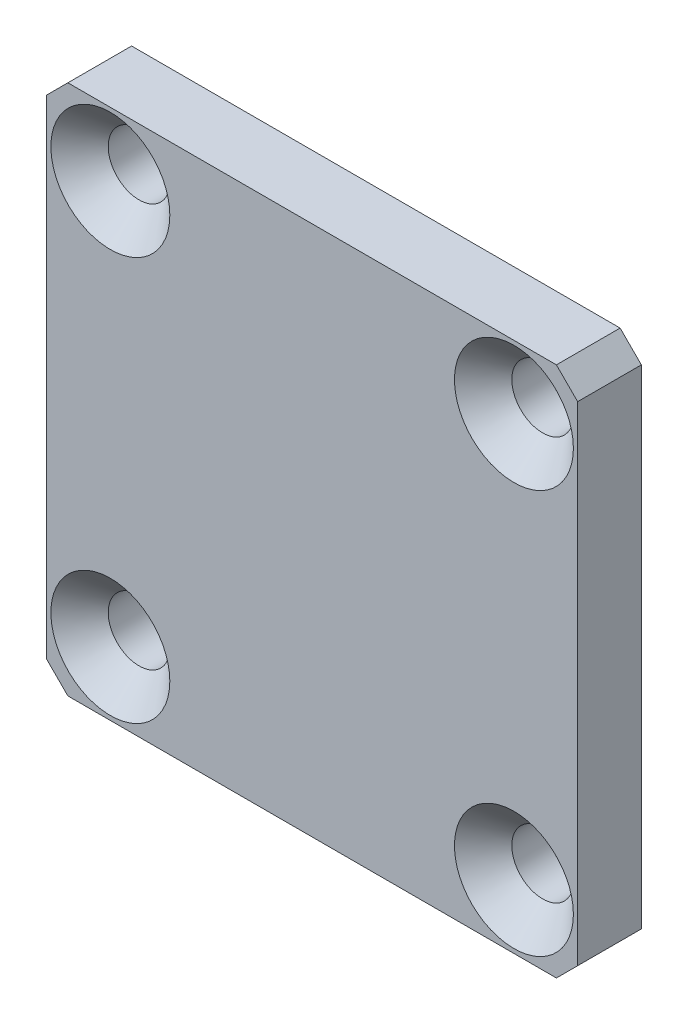
SolidWorks part; units mm, degrees
material "6061Al"
ref_plane "前视基准面" through (0, 0, 0) normal (0, 0, 1) x (1, 0, 0)
ref_plane "上视基准面" through (0, 0, 0) normal (0, 1, 0) x (1, 0, 0)
ref_plane "右视基准面" through (0, 0, 0) normal (1, 0, 0) x (0, 0, -1)
sketch "草图1" plane through (0, 0, 0) normal (0, 0, 1) x (1, 0, 0)
  line L1 (-25, -25) -> (25, -25)
  line L2 (-25, -25) -> (-25, 25)
  line L3 (-25, 25) -> (25, 25)
  line L4 (25, -25) -> (25, 25)
  line L5 (-25, -25) -> (25, 25) construction
  line L6 (-25, 25) -> (25, -25) construction
  point P0 (0, 0)
  dimension "D1" = 50
  dimension "D2" = 50
extrude "凸台-拉伸1" add sketch "草图1" along normal mid plane 6
sketch "草图2" plane through (0, 0, 3) normal (0, 0, 1) x (1, 0, 0)
  circle A0 centre (0, 0) radius 20
  dimension "D1" = 40
extrude "切除-拉伸1" [suppressed] cut sketch "草图2" against normal through all
hole_wizard "M5 六角凹锥坑螺钉的锥形沉头孔1" positions "草图6" profile "草图5" countersink size "M5" standard "ISO" end condition through all
sketch "草图6" plane through (0, 0, 3) normal (0, 0, 1) x (1, 0, 0)
  line L1 (-19, -19) -> (19, -19)
  line L2 (-19, -19) -> (-19, 19)
  line L3 (-19, 19) -> (19, 19)
  line L4 (19, -19) -> (19, 19)
  line L5 (-19, -19) -> (19, 19) construction
  line L6 (-19, 19) -> (19, -19) construction
  line L7 (-25, 25) -> (-25, -25) construction
  point P0 (-19, 19)
  point P4 (19, 19)
  point P7 (-19, -19)
  point P9 (19, -19)
  dimension "D1" = 6
sketch "草图5" plane through (-19, 19, 3) normal (1, 0, 0) x (0, -1, 0)
  line L0 (0, 0) -> (0, 6)
  line L1 (0, 6) -> (2.9, 6)
  line L2 (2.9, 6) -> (2.9, 2.7)
  line L3 (2.9, 2.7) -> (5.6, 0)
  line L5 (5.6, 0) -> (0, 0)
  line L6 (-2.9, 2.7) -> (-5.6, 0) construction
  line L11 (0, -6.35) -> (0, 107.95) construction
  dimension "通孔孔直径" = 5.8
  dimension "通孔孔深度" = 6
  dimension "近端锥形沉头孔直径" = 11.2
  dimension "近端锥形沉头孔角度" = 90
chamfer "倒角1" distance 2 angle 45 4 edges at (-25, -25, 0) (25, -25, 0) (25, 25, 0) (-25, 25, 0)
sketch "草图7" [suppressed] plane through (0, 0, 5) normal (0, 0, 1) x (1, 0, 0)
  circle A0 centre (0, 0) radius 20 construction
  circle A1 centre (0, 0) radius 20
  circle A2 centre (0, 0) radius 12.5
  dimension "D1" = 25
extrude "凸台-拉伸2" [suppressed] add sketch "草图7" against normal blind 3.2
sketch "草图8" plane through (0, 0, -3) normal (0, 0, -1) x (-1, 0, 0)
  circle A0 centre (0, 0) radius 18 construction
  circle A1 centre (0, 0) radius 19.2
  circle A2 centre (0, 0) radius 16.8
  dimension "D1" = 36
  dimension "D2" = 1.2
  dimension "D3" = 1.2
extrude "切除-拉伸2" cut sketch "草图8" against normal blind 1.5
